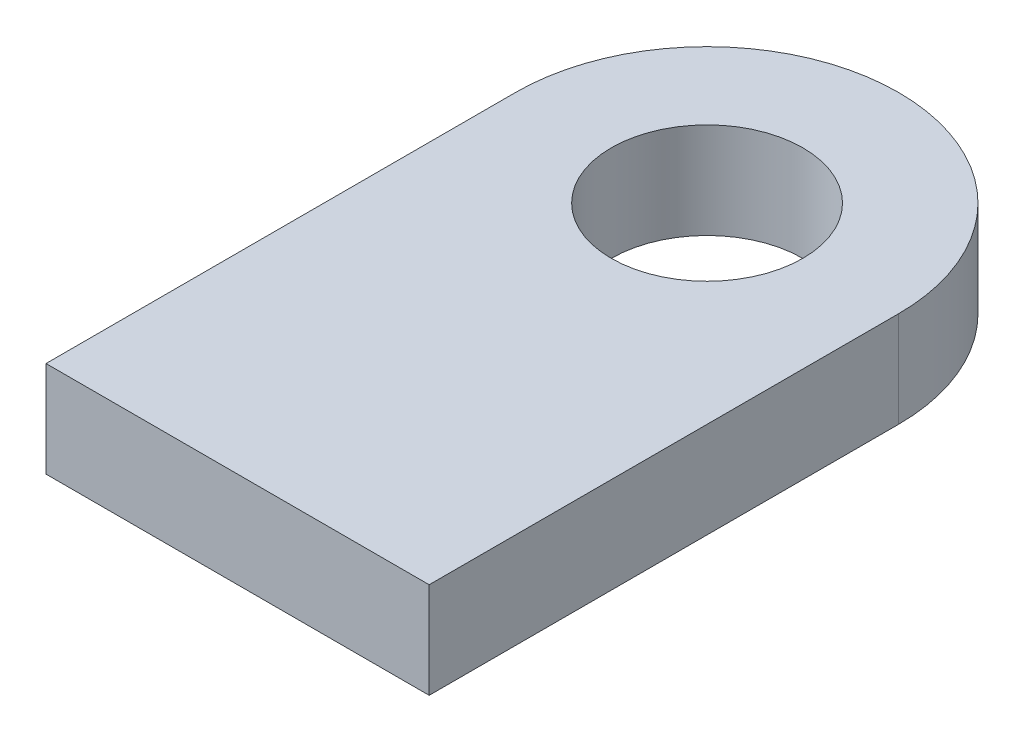
SolidWorks part; units mm, degrees
ref_plane "前视基准面" through (0, 0, 0) normal (0, 0, 1) x (1, 0, 0)
ref_plane "上视基准面" through (0, 0, 0) normal (0, 1, 0) x (1, 0, 0)
ref_plane "右视基准面" through (0, 0, 0) normal (1, 0, 0) x (0, 0, -1)
sketch "草图1" plane through (0, 0, 0) normal (0, 1, 0) x (1, 0, 0)
  line L1 (-20, -24.505) -> (20, -24.505)
  line L2 (-20, -24.505) -> (-20, 24.505)
  line L4 (20, -24.505) -> (20, 24.505)
  line L5 (-20, -24.505) -> (20, 24.505) construction
  line L6 (-20, 24.505) -> (20, -24.505) construction
  arc A1 (20, 24.505) -> (-20, 24.505) centre (0, 24.505) ccw
  circle A2 centre (0, 24.505) radius 10
  point P0 (0, 0)
  dimension "D3" = 20
  dimension "D5" = 20
  dimension "D2" = 40
  dimension "D4" = 49.01
extrude "凸台-拉伸1" add sketch "草图1" along normal mid plane 10
